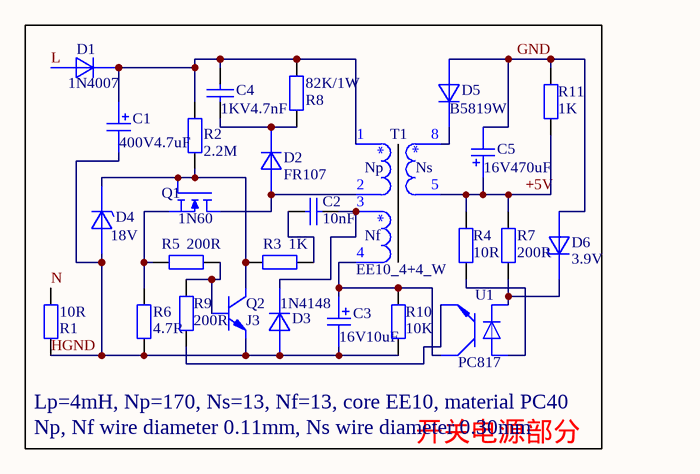
[diagram p0: MISC95139.SchDoc]
# Altium project MISC95139.PrjPcb
1 sheet, 26 parts. Net scope: global (net labels, ports and power ports of the same name join across sheets).
Board file: MISC95139.PcbDoc

## Sheet MISC95139.SchDoc
size A4

### Parts
C1  400V4.7uF  [cap-8*14mm]
C2  10nF  [0805_Cap]
C3  16V10uF  [0805_Cap]
C4  1KV4.7nF  [CAP_5mm]
C5  16V470uF  [cap-8*14mm]
D1  1N4007  [SOD-123]
D2  FR107  [SOD-123]
D3  1N4148  [SOD-123]
D4  18V  [SOD-123]
D5  B5819W  [SOD-123]
D6  3.9V  [SOD-123]
Q1  1N60  [TO-126]
Q2  J3  [SOT23]
R1  10R  [0805_Res]
R2  2.2M  [0805_Res]
R3  1K  [0805_Res]
R4  10R  [0805_Res]
R5  200R  [0805_Res]
R6  4.7R  [0805_Res]
R7  200R  [0805_Res]
R8  82K/1W  [1W_Res_L]
R9  200R  [0805_Res]
R10  10K  [0805_Res]
R11  1K  [0805_Res]
T1  EE10_4+4_W  [EE10_4+4_W]
U1  PC817  [SOP4-PC817]

### Nets
+5V: C5.1 R4.1 R7.2 R11.2 T1.5
GND: C5.2 D5.1(A) D6.1(A) R11.1
HGND: C1.2 C3.2 D3.1(A) D4.1(A) Q2.2(E) R1.2 R6.2 R10.2
L: D1.1(A)
N: R1.1
NetC1_1: C1.1 C4.1 D1.2(K) R2.1 R8.1 T1.1
NetC2_1: C2.1 D3.2(K) T1.3
NetC2_2: C2.2 R3.2
NetC3_1: C3.1 R10.1 T1.4 U1.4
NetC4_2: C4.2 D2.2(K) R8.2
NetD2_1: D2.1(A) Q1.2(D) T1.2
NetD4_2: D4.2(K) Q1.1(G) Q2.3(C) R2.2 R3.1
NetD5_2: D5.2(K) T1.8
NetD6_2: D6.2(K) R7.1 U1.2
NetQ1_3: Q1.3(S) R5.2 R6.1
NetQ2_1: Q2.1(B) R5.1 R9.2
NetR4_2: R4.2 U1.1
NetR9_1: R9.1 U1.3

### Notes on the sheet
- (near T1) Np
- (near T1) Ns
- (near T1) Nf
- Lp=4mH, Np=170, Ns=13, Nf=13, core EE10, material PC40
- Np, Nf wire diameter 0.11mm, Ns wire diameter 0.30mm
- 开关电源部分

### Library data of the parts
C1 C3 C5 = Cap Pol
C2 C4 = Cap: Capacitor; Value: 100pF; Published: 8-Jun-2000; LatestRevisionDate: 17-Jul-2002; LatestRevisionNote: Re-released for DXP Platform.; PackageReference: RAD-0.3; Publisher: Altium Limited
D1-D3 D5 = Diode
D4 D6 = DZener
Q1 = FQPF20N60C: 600V 20A N-Channel MOSFET
Q2 = J3: SMD 9013 NPN-Transistor Vceo=25V,Icm=0.5A
R1 R2 R4-R10 = Res2: Resistor; Value: 1K; Published: 8-Jun-2000; LatestRevisionDate: 17-Jul-2002; LatestRevisionNote: Re-released for DXP Platform.; PackageReference: AXIAL-0.4; Publisher: Altium Limited
R3 R11 = Res2: Resistor; Published: 8-Jun-2000; LatestRevisionDate: 17-Jul-2002; LatestRevisionNote: Re-released for DXP Platform.; PackageReference: AXIAL-0.4; Value: 1K; Publisher: Altium Limited
T1 = Flyback transformer-1
U1 = PC817: Device Specification For PhotoCoupler